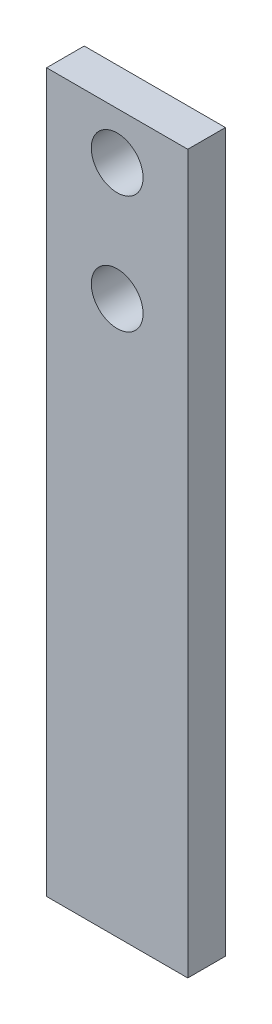
from build123d import *

# Parameters (mm, degrees)
SKETCH_1_W      = 60
SKETCH_1_H      = 305
SKETCH_1_R      = 11
EXTRUDE_1_DEPTH = 8


with BuildPart() as part:
    # 草图1 → 凸台-拉伸1 (new, symmetric)
    with BuildSketch(Plane.XY):
        Rectangle(SKETCH_1_W, SKETCH_1_H)
        with Locations((0, 132.5)):
            Circle(SKETCH_1_R, mode=Mode.SUBTRACT)
        with Locations((0, 82.5)):
            Circle(SKETCH_1_R, mode=Mode.SUBTRACT)
    extrude(amount=EXTRUDE_1_DEPTH, both=True)


solid = part.part
